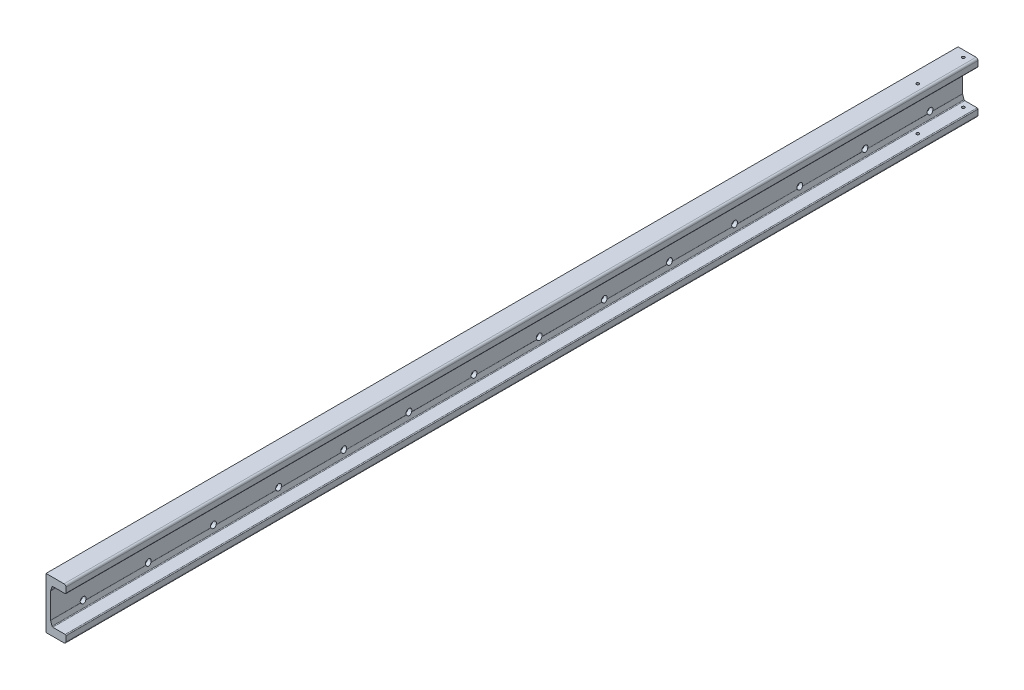
SolidWorks part; units mm, degrees
material "1023 碳钢板 (SS)"
ref_plane "前视基准面" through (0, 0, 0) normal (0, 0, 1) x (1, 0, 0)
ref_plane "上视基准面" through (0, 0, 0) normal (0, 1, 0) x (1, 0, 0)
ref_plane "右视基准面" through (0, 0, 0) normal (1, 0, 0) x (0, 0, -1)
sketch "草图1" plane through (0, 0, 0) normal (0, 0, 1) x (1, 0, 0)
  line L0 (0, 0) -> (-61.2, 0)
  line L1 (-61.2, 0) -> (-61.2, -157.2)
  line L2 (-61.2, -157.2) -> (0, -157.2)
  line L3 (0, -157.2) -> (0, -132.8)
  line L4 (0, -132.8) -> (-42.2, -132.8)
  line L5 (-47.2, -117.8) -> (-47.2, -39.4)
  line L6 (-42.2, -24.4) -> (0, -24.4)
  line L7 (0, -24.4) -> (0, 0)
  line L8 (-47.2, -117.8) -> (-42.2, -132.8)
  line L9 (-61.2, -78.6) -> (-16.126, -78.6) construction
  line L10 (-47.2, -39.4) -> (-42.2, -24.4)
  dimension "D1" = 157.2
  dimension "D2" = 24.4
  dimension "D3" = 108.4
  dimension "D4" = 61.2
  dimension "D5" = 14
  dimension "D6" = 15
extrude "凸台-拉伸1" add sketch "草图1" along normal blind 2800 contours L6 L7 L0 L1 L2 L3 L4 L8 L5 L10
fillet "圆角1" radius 6 2 edges at (0, -157.2, 1400) (0, 0, 1400)
fillet "圆角2" radius 2.5 6 edges at (-42.2, -132.8, 1400) (-47.2, -117.8, 1400) (-47.2, -39.4, 1400) (-42.2, -24.4, 1400) (0, -132.8, 1400) (0, -24.4, 1400)
sketch "草图2" plane through (-61.2, 0, 0) normal (-1, 0, 0) x (0, 0, 1)
  line L0 (0, 0) -> (0, -157.2) construction
  circle A0 centre (100, -113.6) radius 5.5
  circle A1 centre (100, -43.6) radius 5.5
  circle A2 centre (300, -43.6) radius 5.5
  circle A3 centre (300, -113.6) radius 5.5
  circle A4 centre (500, -43.6) radius 5.5
  circle A5 centre (500, -113.6) radius 5.5
  circle A6 centre (700, -43.6) radius 5.5
  circle A7 centre (700, -113.6) radius 5.5
  circle A8 centre (900, -43.6) radius 5.5
  circle A9 centre (900, -113.6) radius 5.5
  circle A10 centre (1100, -43.6) radius 5.5
  circle A11 centre (1100, -113.6) radius 5.5
  circle A12 centre (1300, -43.6) radius 5.5
  circle A13 centre (1300, -113.6) radius 5.5
  circle A14 centre (1500, -43.6) radius 5.5
  circle A15 centre (1500, -113.6) radius 5.5
  circle A16 centre (1700, -43.6) radius 5.5
  circle A17 centre (1700, -113.6) radius 5.5
  circle A18 centre (1900, -43.6) radius 5.5
  circle A19 centre (1900, -113.6) radius 5.5
  circle A20 centre (2100, -43.6) radius 5.5
  circle A21 centre (2100, -113.6) radius 5.5
  circle A22 centre (2300, -43.6) radius 5.5
  circle A23 centre (2300, -113.6) radius 5.5
  circle A24 centre (2500, -43.6) radius 5.5
  circle A25 centre (2500, -113.6) radius 5.5
  circle A26 centre (2700, -43.6) radius 5.5
  circle A27 centre (2700, -113.6) radius 5.5
  point P7 (0, -78.6)
  dimension "D1" = 11
  dimension "D2" = 11
  dimension "D3" = 100
  dimension "D5" = 35
  dimension "D6" = 14
  dimension "D4" = 70
extrude "切除-拉伸1" cut sketch "草图2" against normal blind 3
sketch "草图3" plane through (-58.2, 0, 0) normal (-1, 0, 0) x (0, 0, 1)
  circle A0 centre (100, -43.6) radius 9
  circle A1 centre (100, -113.6) radius 9
  circle A2 centre (300, -43.6) radius 9
  circle A3 centre (300, -113.6) radius 9
  circle A4 centre (500, -43.6) radius 9
  circle A5 centre (500, -113.6) radius 9
  circle A6 centre (700, -43.6) radius 9
  circle A7 centre (700, -113.6) radius 9
  circle A8 centre (900, -43.6) radius 9
  circle A9 centre (900, -113.6) radius 9
  circle A10 centre (1100, -43.6) radius 9
  circle A11 centre (1100, -113.6) radius 9
  circle A12 centre (1300, -43.6) radius 9
  circle A13 centre (1300, -113.6) radius 9
  circle A14 centre (1500, -43.6) radius 9
  circle A15 centre (1500, -113.6) radius 9
  circle A16 centre (1700, -43.6) radius 9
  circle A17 centre (1700, -113.6) radius 9
  circle A18 centre (1900, -43.6) radius 9
  circle A19 centre (1900, -113.6) radius 9
  circle A20 centre (2100, -43.6) radius 9
  circle A21 centre (2100, -113.6) radius 9
  circle A22 centre (2300, -43.6) radius 9
  circle A23 centre (2300, -113.6) radius 9
  circle A24 centre (2500, -43.6) radius 9
  circle A25 centre (2500, -113.6) radius 9
  circle A26 centre (2700, -43.6) radius 9
  circle A27 centre (2700, -113.6) radius 9
  dimension "D1" = 18
  dimension "D2" = 18
  dimension "D3" = 14
extrude "切除-拉伸2" cut sketch "草图3" against normal blind 31
sketch "草图4" plane through (0, 0, 0) normal (0, 1, 0) x (1, 0, 0)
  line L0 (0, 0) -> (0, -2800) construction
  line L1 (-6, 0) -> (-61.2, 0) construction
  circle A0 centre (-25, -20) radius 5
  circle A1 centre (-25, -160) radius 5
  dimension "D2" = 20
  dimension "D4" = 10
  dimension "D5" = 10
  dimension "D1" = 25
  dimension "D3" = 140
hole_wizard "M10 螺纹孔1" positions "草图5" profile "草图6" tap size "M10" standard "ISO" end condition through all
sketch "草图5" plane through (0, 0, 0) normal (0, 1, 0) x (1, 0, 0)
  point P0 (-25, -20)
  point P3 (-25, -160)
sketch "草图6" plane through (-25, 0, 20) normal (1, 0, 0) x (0, 0, 1)
  line L0 (0, 0) -> (0, 157.2)
  line L1 (0, 157.2) -> (4.25, 157.2)
  line L2 (4.25, 157.2) -> (4.25, 0)
  line L5 (4.25, 0) -> (0, 0)
  line L11 (0, -6.35) -> (0, 107.95) construction
  dimension "通孔螺纹孔钻头直径" = 8.5
  dimension "通孔螺纹孔钻头深度" = 157.2
cosmetic thread "孔螺蚊线1" parameters "D2"=10
cosmetic thread "孔螺蚊线2" parameters "D2"=10
